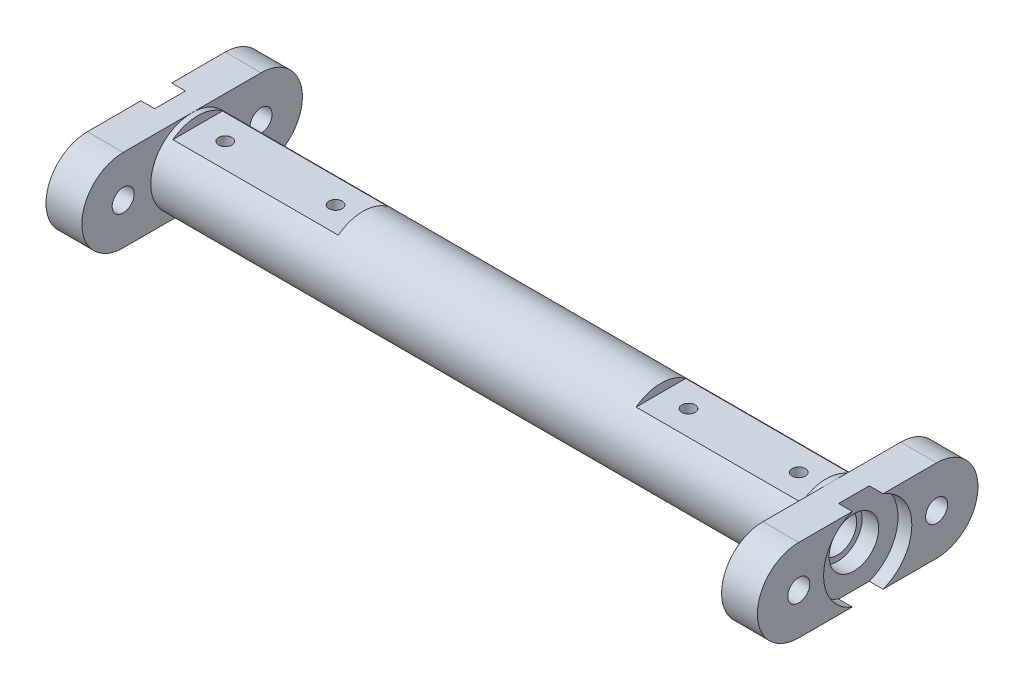
SolidWorks part; units mm, degrees
ref_plane "Front Plane" through (0, 0, 0) normal (0, 0, 1) x (1, 0, 0)
ref_plane "Top Plane" through (0, 0, 0) normal (0, 1, 0) x (1, 0, 0)
ref_plane "Right Plane" through (0, 0, 0) normal (1, 0, 0) x (0, 0, -1)
sketch "Sketch 1" plane through (0, 0, 0) normal (0, 0, 1) x (1, 0, 0)
  line L0 (0, 323.4127) -> (0, -351.1905) construction
  line L1 (-862.8571, 0) -> (882.8571, 0) construction
  line L2 (590, 35) -> (-590, 35)
  line L3 (-590, 35) -> (-590, 45)
  line L4 (-590, 45) -> (-620, 45)
  line L5 (-620, 45) -> (-620, 75)
  line L6 (-620, 75) -> (620, 75)
  line L7 (620, 45) -> (620, 75)
  line L8 (590, 45) -> (620, 45)
  line L9 (590, 35) -> (590, 45)
  point P13 (0, 75)
  point P16 (0, 35)
  dimension "D1" = 1240
  dimension "D2" = 90
  dimension "D3" = 150
  dimension "D4" = 30
  dimension "D5" = 70
revolve "Revolve 1" add sketch "Sketch 1" angle 360 about L1
sketch "Sketch 2" plane through (0, 0, 0) normal (0, 0, 1) x (1, 0, 0)
  line L0 (0, 265.6934) -> (0, -245.2555) construction
  line L1 (620, 75) -> (-620, 75) construction
  line L2 (-570, 75) -> (-270, 75)
  line L3 (-570, 75) -> (-570, 60)
  line L4 (-570, 60) -> (-270, 60)
  line L5 (-270, 75) -> (-270, 60)
  line L6 (-731.4895, 0) -> (77.752, 0) construction
  line L7 (270, 75) -> (270, 60)
  line L8 (570, 60) -> (270, 60)
  line L9 (570, 75) -> (570, 60)
  line L10 (570, 75) -> (270, 75)
  line L11 (-420, 75) -> (-420, 29.0519) construction
  dimension "D1" = 300
  dimension "D2" = 420
  dimension "D3" = 60
extrude "Cut-Extrude 1" cut sketch "Sketch 2" against normal through all both and the other way through all
sketch "Sketch 3" plane through (0, 60, 0) normal (0, 1, 0) x (1, 0, 0)
  line L0 (0, 142.6864) -> (0, -176.6226) construction
  line L1 (-420, 45) -> (-420, -45) construction
  line L2 (-570, 45) -> (-270, 45) construction
  line L3 (-270, -45) -> (-570, -45) construction
  line L4 (-765.1075, 0) -> (-206.7024, 0) construction
  circle A0 centre (-320, 0) radius 12
  circle A1 centre (-520, 0) radius 12
  circle A2 centre (520, 0) radius 12
  circle A3 centre (320, 0) radius 12
  dimension "D1" = 100
  dimension "D2" = 24
extrude "Cut-Extrude 2" cut sketch "Sketch 3" against normal up to surface (25 mm away)
sketch "Sketch 4" plane through (-620, 0, 0) normal (-1, 0, 0) x (0, 0, 1)
  line L0 (-204.25, 0) -> (206.3342, 0) construction
  line L1 (-125, 0) -> (125, 0) construction
  line L2 (-125, 75) -> (125, 75)
  line L3 (-125, -75) -> (125, -75)
  line L4 (0, 96.133) -> (0, -101.3434) construction
  arc A0 (-125, 75) -> (-125, -75) centre (-125, 0) ccw
  arc A1 (125, -75) -> (125, 75) centre (125, 0) ccw
  circle A2 centre (0, 0) radius 75 construction
  circle A3 centre (-125, 0) radius 20
  circle A4 centre (125, 0) radius 20
  circle A7 centre (0, 0) radius 45 construction
  circle A8 centre (0, 0) radius 45
  point P5 (0, 0)
  dimension "D1" = 40
  dimension "D2" = 250
extrude "Boss-Extrude 1" add sketch "Sketch 4" against normal blind 40
sketch "Sketch 5" plane through (-620, 0, 0) normal (-1, 0, 0) x (0, 0, 1)
  line L0 (0, 104.2034) -> (0, -105.0664) construction
  line L1 (-27.8388, 75) -> (-125, 75)
  line L3 (125, 75) -> (-125, 75)
  line L4 (-125, -75) -> (125, -75)
  line L6 (-125, -75) -> (-27.8388, -75)
  line L8 (125, 75) -> (-125, 75) construction
  line L9 (125, -75) -> (27.8388, -75)
  line L10 (27.8388, 75) -> (125, 75)
  circle A1 centre (-125, 0) radius 20 construction
  circle A2 centre (-125, 0) radius 20
  arc A3 (125, -75) -> (125, 75) centre (125, 0) ccw
  arc A4 (-125, 75) -> (-125, -75) centre (-125, 0) ccw
  arc A6 (-125, 75) -> (-125, -75) centre (-125, 0) ccw
  arc A7 (-27.8388, 75) -> (-27.8388, -75) centre (0, 0) ccw
  arc A10 (-125, 75) -> (-125, -75) centre (-125, 0) ccw construction
  arc A11 (27.8388, 75) -> (27.8388, -75) centre (0, 0) cw
  arc A12 (125, 75) -> (125, -75) centre (125, 0) cw
  circle A13 centre (125, 0) radius 20
  dimension "D2" = 160
  dimension "D1" = 0
extrude "Boss-Extrude 2" add sketch "Sketch 5" along normal blind 25
mirror "Mirror 1" about plane through (0, 0, 0) normal (1, 0, 0) of "Boss-Extrude 2", "Boss-Extrude 1"
